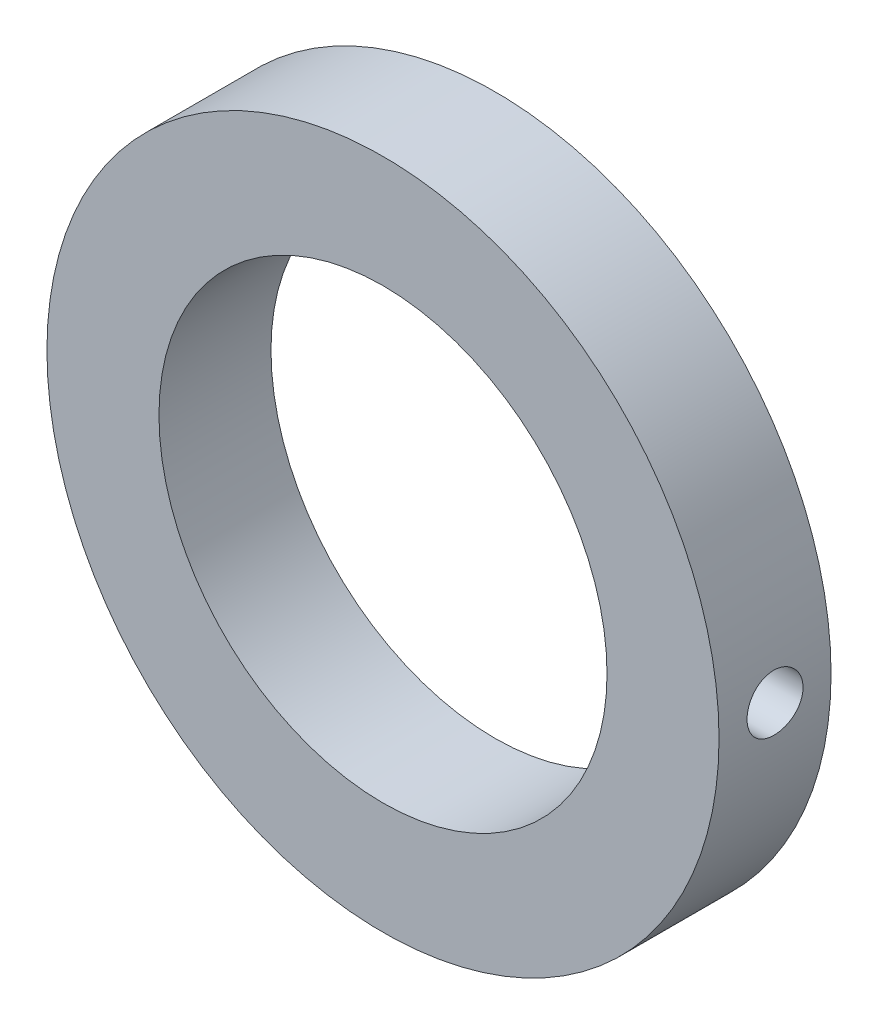
from build123d import *

# Parameters (mm, degrees)
SKETCH_1_R             = 15
SKETCH_1_R_2           = 10
EXTRUDE_1_DEPTH        = 5
HOLE_WIZARD_M3_2_D     = 2.5
HOLE_WIZARD_M3_2_DEPTH = 7.5
HOLE_WIZARD_M3_2_TIP   = 0.751075774


with BuildPart() as part:
    # 草图1 → 凸台-拉伸1 (new body)
    with BuildSketch(Plane.XY):
        Circle(SKETCH_1_R)
        Circle(SKETCH_1_R_2, mode=Mode.SUBTRACT)
    extrude(amount=EXTRUDE_1_DEPTH)

    # M3 螺纹孔2
    with Locations(Plane(origin=(14.999656228, 0.101553124, 2.5), x_dir=(-0.006770208298, 0.999977081877, 0), z_dir=(0.999977081877, 0.006770208298, 0))):
        with Locations((0, 0)):
            Hole(HOLE_WIZARD_M3_2_D / 2, depth=HOLE_WIZARD_M3_2_DEPTH)
            with Locations((0, 0, -(HOLE_WIZARD_M3_2_DEPTH + HOLE_WIZARD_M3_2_TIP / 2))):  # 118° drill point
                Cone(0, HOLE_WIZARD_M3_2_D / 2, HOLE_WIZARD_M3_2_TIP, mode=Mode.SUBTRACT)


solid = part.part
